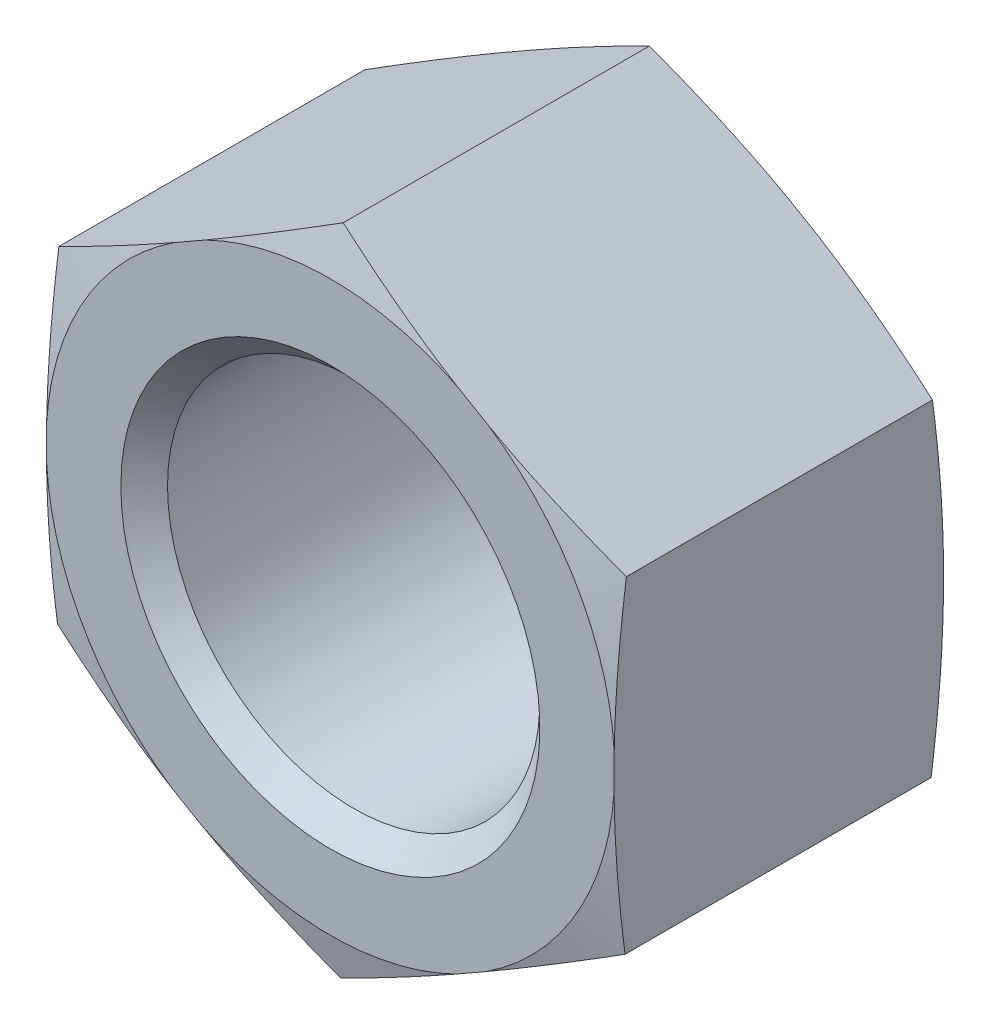
from build123d import *

# Parameters (mm, degrees)
SKETCH1_R          = 18.4
BASE_EXTRUDE_DEPTH = 32.54375
SKETCH2_OUTSIDE_W  = 485.848
SKETCH2_OUTSIDE_H  = 494.398
SKETCH2_OUTSIDE_R  = 28.1
CUT_EXTRUDE1_DEPTH = 54.833293767
CUT_EXTRUDE1_DRAFT = -75
SKETCH3_OUTSIDE_W  = 485.848
SKETCH3_OUTSIDE_H  = 494.398
SKETCH3_OUTSIDE_R  = 28.1
CUT_EXTRUDE2_DEPTH = 54.833293767
CUT_EXTRUDE2_DRAFT = -75
CHAMFER1_SIZE      = 2.307142857


with BuildPart() as part:
    # Sketch1 → Base-Extrude (new body)
    with BuildSketch(Plane.XY):
        Polygon((0.127390736, 32.384749445), (-27.982320346, 16.302698336), (-28.109711083, -16.082051108), (-0.127390736, -32.384749445), (27.982320346, -16.302698336), (28.109711083, 16.082051108), align=None)
        Circle(SKETCH1_R, mode=Mode.SUBTRACT)
    extrude(amount=BASE_EXTRUDE_DEPTH)


with BuildPart() as cut_extrude1_tool:
    # Sketch2 outside → Cut-Extrude1 (with draft: the straight prism first)
    with BuildSketch(Plane(origin=(0, 0, 0), x_dir=(-1, 0, 0), z_dir=(0, 0, -1))):
        Rectangle(SKETCH2_OUTSIDE_W, SKETCH2_OUTSIDE_H)
        Circle(SKETCH2_OUTSIDE_R, mode=Mode.SUBTRACT)
    extrude(amount=-CUT_EXTRUDE1_DEPTH)
    # Cut-Extrude1: the draft: its side faces are tilted about the plane it starts from
    cut_extrude1_sides = [cut_extrude1_tool.faces().sort_by_distance(p)[0] for p in [
        (0, -247.199, 27.416646884),
        (-242.924, 0, 27.416646884),
        (0, 247.199, 27.416646884),
        (242.924, 0, 27.416646884),
        (28.1, 0, 27.416646884),
    ]]
    draft(cut_extrude1_sides, Plane(origin=(0, 0, 0), x_dir=(-1, 0, 0), z_dir=(0, 0, -1)), CUT_EXTRUDE1_DRAFT)


with BuildPart() as part_1:
    add(part.part)

    # Cut-Extrude1: cut by cut_extrude1_tool
    add(cut_extrude1_tool.part, mode=Mode.SUBTRACT)


with BuildPart() as cut_extrude2_tool:
    # Sketch3 outside → Cut-Extrude2 (with draft: the straight prism first)
    with BuildSketch(Plane.XY.offset(32.54375)):
        Rectangle(SKETCH3_OUTSIDE_W, SKETCH3_OUTSIDE_H)
        Circle(SKETCH3_OUTSIDE_R, mode=Mode.SUBTRACT)
    extrude(amount=-CUT_EXTRUDE2_DEPTH)
    # Cut-Extrude2: the draft: its side faces are tilted about the plane it starts from
    cut_extrude2_sides = [cut_extrude2_tool.faces().sort_by_distance(p)[0] for p in [
        (0, -247.199, 5.127103116),
        (242.924, 0, 5.127103116),
        (0, 247.199, 5.127103116),
        (-242.924, 0, 5.127103116),
        (-28.1, 0, 5.127103116),
    ]]
    draft(cut_extrude2_sides, Plane.XY.offset(32.54375), CUT_EXTRUDE2_DRAFT)


with BuildPart() as part_2:
    add(part_1.part)

    # Cut-Extrude2: cut by cut_extrude2_tool
    add(cut_extrude2_tool.part, mode=Mode.SUBTRACT)

    # Chamfer1
    chamfer1_edges = [part_2.edges().sort_by_distance(p)[0] for p in [
        (-18.4, 0, 0),
        (-18.4, 0, 32.54375),
    ]]
    chamfer(chamfer1_edges, length=CHAMFER1_SIZE)


solid = part_2.part
